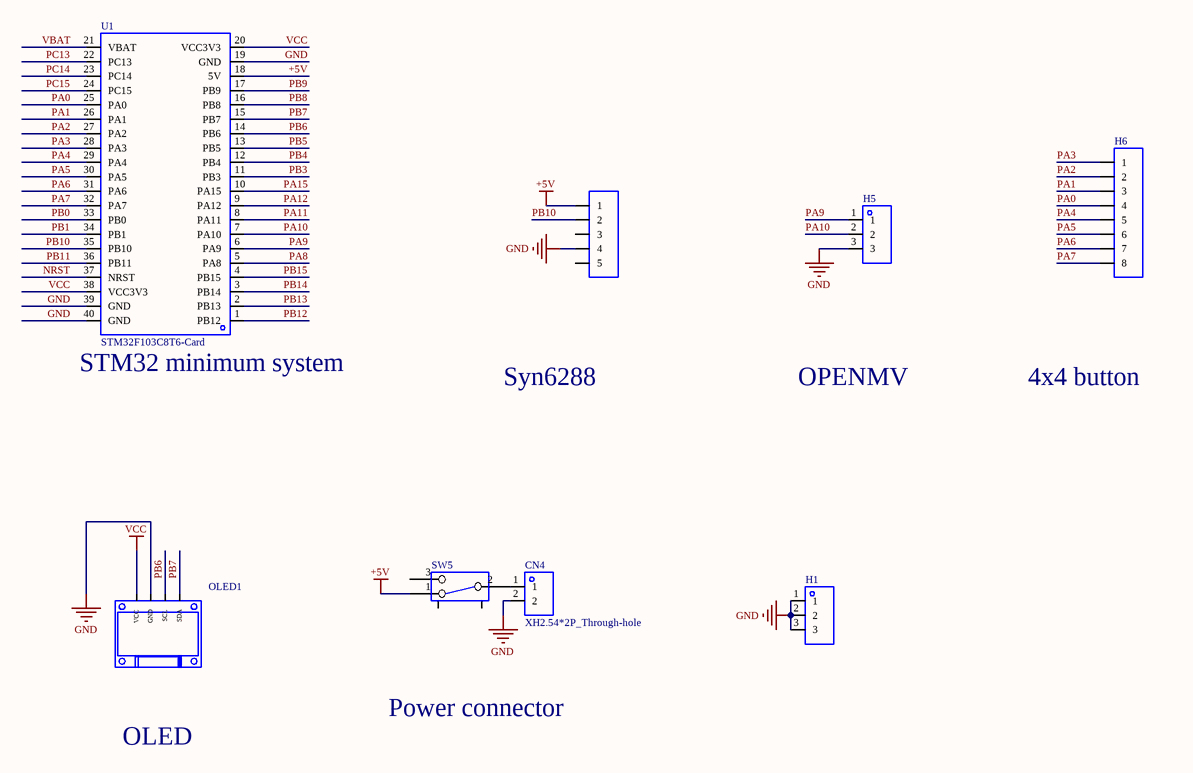
[diagram p0: MISC51713-3.schdoc]
# Altium project MISC51713-2.PrjPcb
1 sheet, 8 parts. Net scope: global (net labels, ports and power ports of the same name join across sheets).
Board file: MISC51713.pcbdoc

## Sheet MISC51713-3.schdoc
size 297 x 209 mm; Version: V1.0; @Project Name: MISC51713; @Page Count: 1; @Update Date: 2026-04-16; @Create Date: 2026-04-16; @Schematic Name: MISC51713; @Page No: 1; @Create Time: 23:22:16; @Update Time: 17:32:40; @Board Name: MISC51713

### Parts
CN4  XH2.54*2P_Through-hole  [CONN-TH_2P-P2.50-XH2.54-2P]
H1  (no value)  [HDR-TH_3P-P2.54-V-M]
H5  (no value)  [HDR-TH_3P-P2.54-V-M]
H6  (no value)  [HDR-TH_8P-P2.54-V-F-1]
OLED1  (no value)  [0.96OLED_4P]
SW5  (no value)  [拨动开关]
U1  STM32F103C8T6-Card  [CONN-TH_L53.3-W22.9_STM32F103C8T6-CARD]
插槽出版子  (no value)  [HDR-TH_5P-P2.54-V-F]

### Nets
+5V: SW5.1 U1.18(5V) 插槽出版子.1
GND: CN4.2 H1.1 H1.2 H1.3 H5.3 OLED1.2(GND) U1.19(GND) U1.39(GND) U1.40(GND) 插槽出版子.4
VCC: OLED1.1(VCC) U1.20(VCC3V3) U1.38(VCC3V3)
NRST: U1.37(NRST)
PA0: H6.4 U1.25(PA0)
PA1: H6.3 U1.26(PA1)
PA2: H6.2 U1.27(PA2)
PA3: H6.1 U1.28(PA3)
PA4: H6.5 U1.29(PA4)
PA5: H6.6 U1.30(PA5)
PA6: H6.7 U1.31(PA6)
PA7: H6.8 U1.32(PA7)
PA8: U1.5(PA8)
PA9: H5.1 U1.6(PA9)
PA10: H5.2 U1.7(PA10)
PA11: U1.8(PA11)
PA12: U1.9(PA12)
PA15: U1.10(PA15)
PB0: U1.33(PB0)
PB1: U1.34(PB1)
PB3: U1.11(PB3)
PB4: U1.12(PB4)
PB5: U1.13(PB5)
PB6: OLED1.3(SCL) U1.14(PB6)
PB7: OLED1.4(SDA) U1.15(PB7)
PB8: U1.16(PB8)
PB9: U1.17(PB9)
PB10: U1.35(PB10) 插槽出版子.2
PB11: U1.36(PB11)
PB12: U1.1(PB12)
PB13: U1.2(PB13)
PB14: U1.3(PB14)
PB15: U1.4(PB15)
PC13: U1.22(PC13)
PC14: U1.23(PC14)
PC15: U1.24(PC15)
VBAT: U1.21(VBAT)
NetCN4_1: CN4.1 SW5.2

Not connected (* = marked no-connect by the designer): SW5 3 4 5; 插槽出版子 3 5

### Notes on the sheet
- (near U1) STM32 minimum system
- Syn6288
- OPENMV
- 4x4 button
- Power connector
- OLED
- 2025-04-07
- Schematic
- Board
- Sheet
- 2025-04-21
- P1
- Drawn
- Reviewed
- .stm32v6
- Revision
- Size
- A4
- page 1 Total 1

### Library data of the parts
CN4 = XH2.54*2P_直插: 3D Model: 325c595e30db4df8abe76612dd40b0fa0819f05c4eef4c71ace90d822a990e87; 3D Model Transform: 295.275,228.346,0,180,0,0,-0.002,-20.079,-137.795; AddInBom: yes; Device: XH2.54*2P_Through-hole; Symbol: XH2.54*2P_Through-hole; LCSC Part Name: XH2.54*2P_直插; Supplier Part: C9900008615; Manufacturer Part: XH2.54*2P_直插; Supplier Footprint: XH2.54_2P; JLCPCB Part Class: Extended Part; Supplier: LCSC; FootprintName: CONN-TH_2P-P2.50-XH2.54-2P; ConvertToPcb: yes; ModelName: CONN-TH_2P-P2.50-XH2.54-2P
H1 = HDR-M_2.54_1x3P: 3D Model: bb473b6d38ff42a99216a4fcdbdcc4cb0819f05c4eef4c71ace90d822a990e87; 3D Model Transform: 300.03877,100,0,0,0,0,0,0,-118.11; AddInBom: yes; ModelName: HDR-TH_3P-P2.54-M-LI-1X3P; Symbol: HDR-M_2.54_1x3P; Device: HDR-M_2.54_1x3P; Supplier Part: C2937625; Supplier Footprint: 插件; ConvertToPcb: yes; FootprintName: HDR-TH_3P-P2.54-V-M
H5 = HDR-M_2.54_1x3P: AddInBom: yes; ModelId: bb473b6d38ff42a99216a4fcdbdcc4cb0819f05c4eef4c71ace90d822a990e87; ModelName: HDR-TH_3P-P2.54-M-LI-1X3P; ModelTransform: 300.03877,100,0,0,0,0,0,0,-118.11; Symbol: HDR-M_2.54_1x3P; Device: HDR-M_2.54_1x3P; ConvertToPcb: yes; FootprintName: HDR-TH_3P-P2.54-V-M; SupplierPart: C2937625; Supplier Footprint: 插件
H6 = HDR-F_2.54_1x8P: Symbol: Header-Female-2.54_1x8; AddInBom: yes; ModelId: 0f7e4d9227ef4fa08d5469c22cc70cdb; ModelName: HDR-F-2.54_1x8; ModelTransform: 799.99844,100,0,0,0,0,0,0,-118.11; Device: HDR-F_2.54_1x8P; ConvertToPcb: yes; FootprintName: HDR-TH_8P-P2.54-V-F-1; SupplierPart: C27438; Supplier Footprint: 插件
OLED1 = 0.96OLED模块_4P: Device: 0.96OLED module_4P; Symbol: 0.96OLED module_4P_1; ConvertToPcb: yes; ModelId: 79c000fdb68d45a296c2e9bedf4f9055; ModelTransform: 1393.69792,1318.895,0,0,0,0,0,-560.079,-137.795; FootprintName: 0.96OLED_4P; AddInBom: yes; Supplier Footprint: 插件; ModelName: 0.96OLED_4P
SW5 = 拨动开关_正: Device: Toggle switch_Pos; Symbol: Toggle switch; ConvertToPcb: yes; ModelId: 4321fe59a4074cbfb4989553f297c68f0819f05c4eef4c71ace90d822a990e87; ModelName: SW-TH_SS-12D02-VG4; ModelTransform: 370.09,208.7,472.35,0,0,0,0,0,-110; FootprintName: Toggle switch; AddInBom: yes; Supplier Footprint: 插件
U1 = STM32F103C8T6-Card: AddInBom: yes; Device: STM32F103C8T6-Card; Symbol: STM32F103C8T6-CARD; FootprintName: CONN-TH_L53.3-W22.9_STM32F103C8T6-CARD; LCSC Part Name: STM32F103C8T6-Card; SupplierPart: C9900077949; ManufacturerPart: STM32F103C8T6-Card; Supplier Footprint: 插件; Supplier: LCSC; ConvertToPcb: yes
插槽出版子 = HDR-F_2.54_1x5P: Symbol: Header-Female-2.54_1x5; ConvertToPcb: yes; ModelId: f49cb6116a3d45e5a64915bf3e00773f; ModelTransform: 519.684,98.464,0,0,0,0,0,0,-124.016; Device: HDR-F_2.54_1x5P; AddInBom: yes; SupplierPart: C50950; Supplier Footprint: 插件; FootprintName: HDR-TH_5P-P2.54-V-F; ModelName: HDR-TH_5P-P2.54-V-F